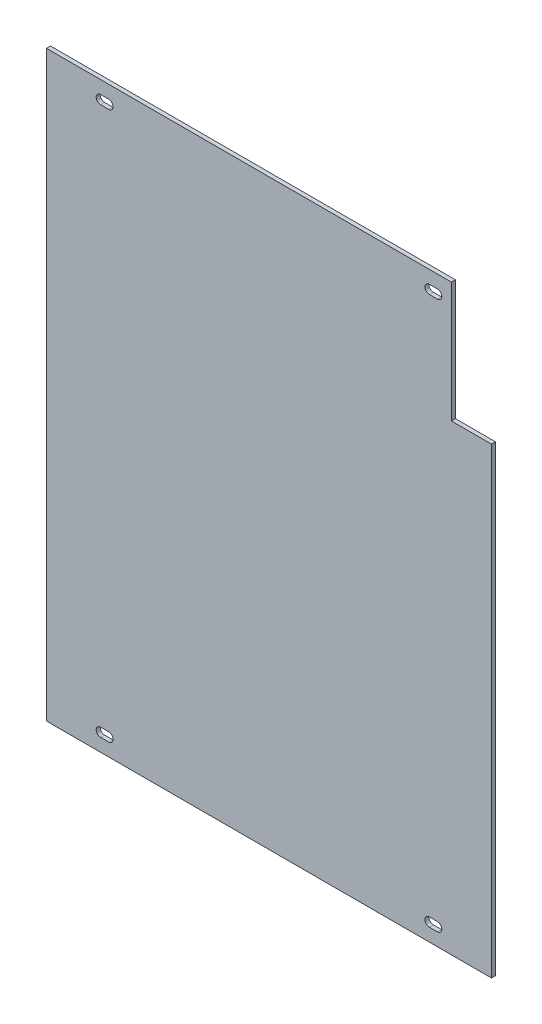
from build123d import *

# Parameters (mm, degrees)
SKETCH_1_W          = 333
SKETCH_1_H          = 436
EXTRUDE_1_DEPTH     = 3
SKETCH_3_W          = 30
SKETCH_3_H          = 90
CUT_EXTRUDE_2_DEPTH = 10
CUT_EXTRUDE_3_DEPTH = 10


with BuildPart() as part:
    # 草图1 → 凸台-拉伸1 (new body)
    with BuildSketch(Plane.XY):
        Rectangle(SKETCH_1_W, SKETCH_1_H)
    extrude(amount=EXTRUDE_1_DEPTH)

    # 草图3 → 切除-拉伸2 (cut)
    with BuildSketch(Plane(origin=(0, 0, 0), x_dir=(-1, 0, 0), z_dir=(0, 0, -1))):
        with Locations((-151.5, 173)):
            Rectangle(SKETCH_3_W, SKETCH_3_H)
    extrude(amount=-CUT_EXTRUDE_2_DEPTH, mode=Mode.SUBTRACT)

    # 草图4 → 切除-拉伸3 (cut)
    with BuildSketch(Plane.XY.offset(3)):
        with BuildLine():
            Line((-120, 201.7), (-126, 201.7))
            ThreePointArc((-126, 201.7), (-129.3, 205), (-126, 208.3))
            Line((-126, 208.3), (-120, 208.3))
            ThreePointArc((-120, 208.3), (-116.7, 205), (-120, 201.7))
        make_face()
        with BuildLine():
            Line((120, 208.3), (126, 208.3))
            ThreePointArc((126, 208.3), (129.3, 205), (126, 201.7))
            Line((126, 201.7), (120, 201.7))
            ThreePointArc((120, 201.7), (116.7, 205), (120, 208.3))
        make_face()
        with BuildLine():
            Line((120, -201.7), (126, -201.7))
            ThreePointArc((126, -201.7), (129.3, -205), (126, -208.3))
            Line((126, -208.3), (120, -208.3))
            ThreePointArc((120, -208.3), (116.7, -205), (120, -201.7))
        make_face()
        with BuildLine():
            Line((-120, -208.3), (-126, -208.3))
            ThreePointArc((-126, -208.3), (-129.3, -205), (-126, -201.7))
            Line((-126, -201.7), (-120, -201.7))
            ThreePointArc((-120, -201.7), (-116.7, -205), (-120, -208.3))
        make_face()
    extrude(amount=-CUT_EXTRUDE_3_DEPTH, mode=Mode.SUBTRACT)


solid = part.part
